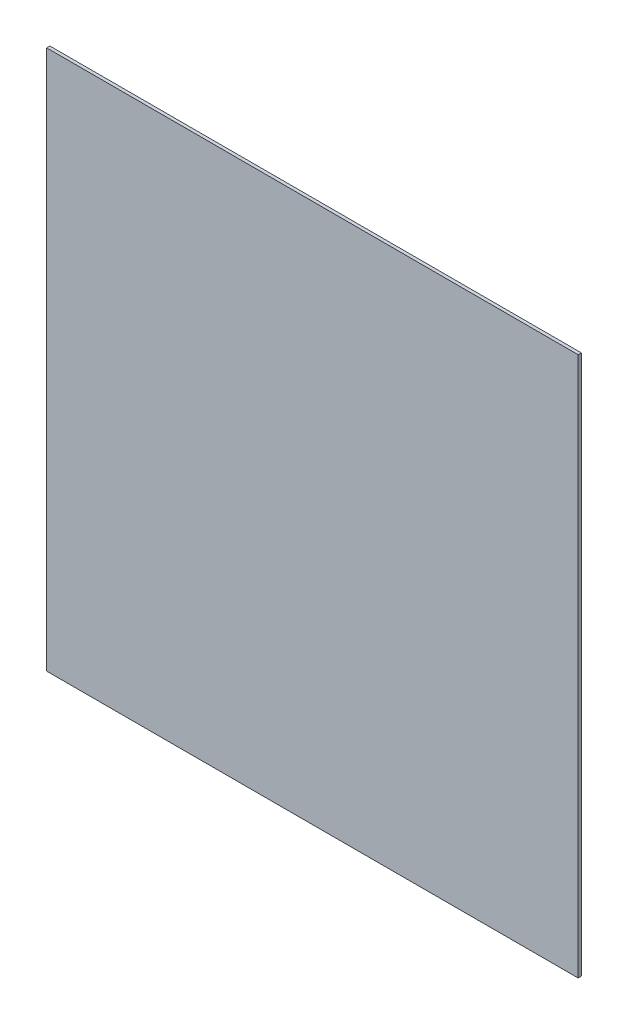
SolidWorks part; units mm, degrees
material "PMMA(有机玻璃)"
ref_plane "前视" through (0, 0, 0) normal (0, 0, 1) x (1, 0, 0)
ref_plane "上视" through (0, 0, 0) normal (0, 1, 0) x (1, 0, 0)
ref_plane "右视" through (0, 0, 0) normal (1, 0, 0) x (0, 0, -1)
sketch "草图1" plane through (0, 0, 0) normal (0, 0, 1) x (1, 0, 0)
  line L1 (-414.5, 421) -> (414.5, 421)
  line L2 (-414.5, 421) -> (-414.5, -421)
  line L3 (-414.5, -421) -> (414.5, -421)
  line L4 (414.5, 421) -> (414.5, -421)
  line L5 (-414.5, 421) -> (414.5, -421) construction
  line L6 (-414.5, -421) -> (414.5, 421) construction
  point P0 (0, 0)
  dimension "D1" = 842
  dimension "D2" = 829
extrude "凸台-拉伸1" add sketch "草图1" along normal blind 5
hole_wizard "M5 间隙孔1" positions "草图3" profile "草图2" hole size "M5" standard "GB"
sketch "草图3" plane through (0, 0, 5) normal (0, 0, 1) x (1, 0, 0)
  line L0 (-427.5, 273) -> (-427.5, -273) construction
  line L1 (-427.5, -273) -> (427.5, -273) construction
  line L2 (0, 273) -> (0, -273) construction
  line L3 (427.5, 273) -> (-427.5, 273) construction
  line L5 (-427.5, 0) -> (427.5, 0) construction
  line L6 (427.5, -273) -> (427.5, 273) construction
  point P0 (-375, -261)
  point P46 (415.5, 250)
  point P48 (-415.5, 250)
  point P58 (-125, -261)
  point P59 (125, -261)
  point P61 (-125, 261)
  point P62 (125, 261)
  point P64 (-375, 261)
  point P88 (375, -261)
  point P89 (375, 261)
  point P108 (415.5, 0)
  point P109 (-415.5, 0)
  point P110 (415.5, -250)
  point P111 (-415.5, -250)
  dimension "D1" = 12
  dimension "D2" = 12
  dimension "D5" = 3
  dimension "D3" = 12
  dimension "D6" = 4
  dimension "D4" = 2
sketch "草图2" plane through (-375, -261, 5) normal (1, 0, 0) x (0, -1, 0)
  line L0 (0, 0) -> (0, 5)
  line L1 (0, 5) -> (2.75, 5)
  line L2 (2.75, 5) -> (2.75, 0)
  line L5 (2.75, 0) -> (0, 0)
  line L11 (0, -6.35) -> (0, 107.95) construction
  dimension "通孔孔直径" = 5.5
  dimension "通孔孔深度" = 5
